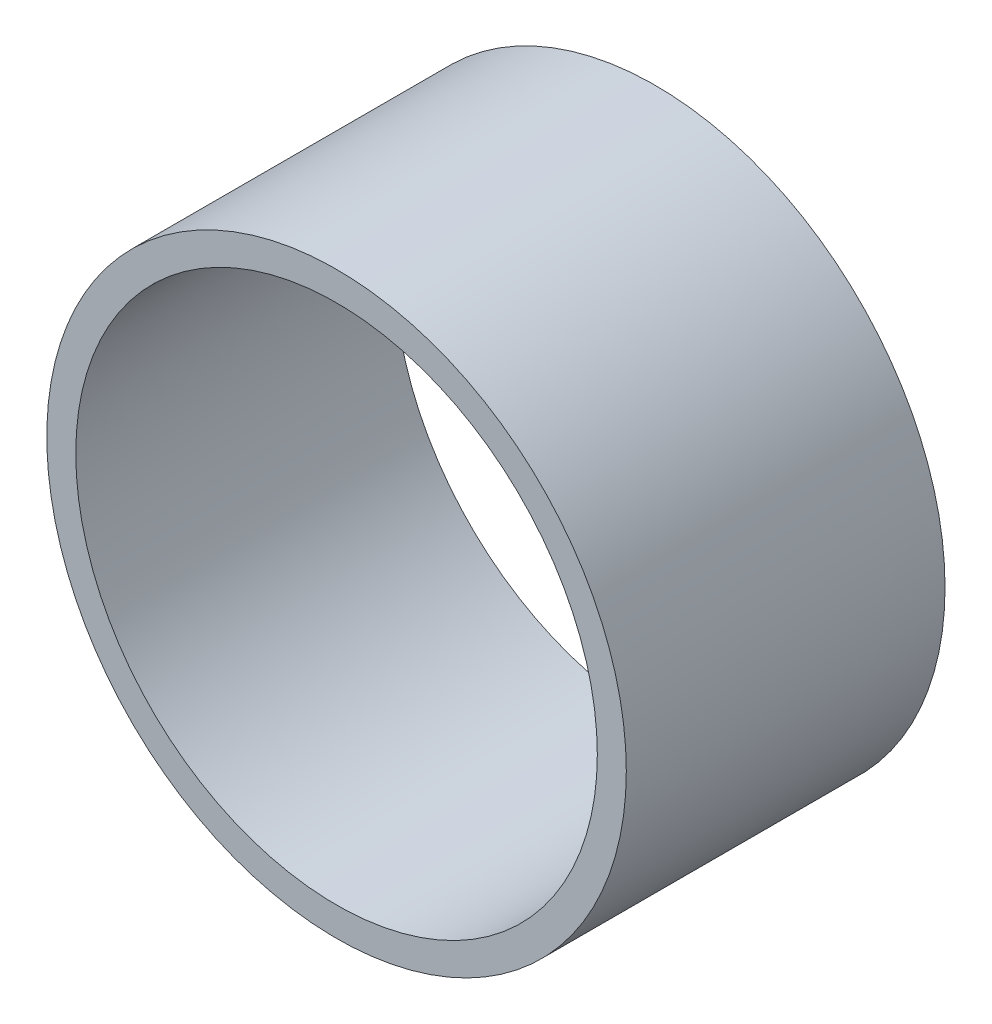
SolidWorks part; units mm, degrees
material "Q235B"
ref_plane "Front Plane" through (0, 0, 0) normal (0, 0, 1) x (1, 0, 0)
ref_plane "Top Plane" through (0, 0, 0) normal (0, 1, 0) x (1, 0, 0)
ref_plane "Right Plane" through (0, 0, 0) normal (1, 0, 0) x (0, 0, -1)
sketch "Sketch1" plane through (0, 0, 0) normal (0, 0, 1) x (1, 0, 0)
  circle A0 centre (-1060, 0) radius 40
  circle A1 centre (-1060, 0) radius 36
  dimension "D1" = 80
  dimension "D2" = 4
extrude "Boss-Extrude1" add sketch "Sketch1" along normal blind 44
